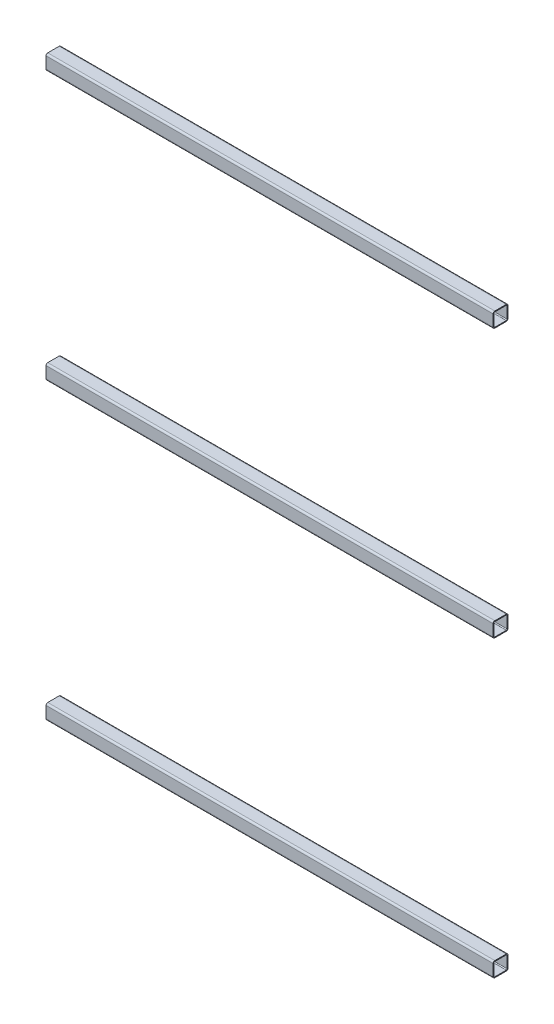
SolidWorks part; units mm, degrees
material "Q235"
ref_plane "Front" through (0, 0, 0) normal (0, 0, 1) x (1, 0, 0)
ref_plane "Top" through (0, 0, 0) normal (0, 1, 0) x (1, 0, 0)
ref_plane "Right" through (0, 0, 0) normal (1, 0, 0) x (0, 0, -1)
sketch "Sketch1" plane through (0, 0, 0) normal (0, 0, 1) x (1, 0, 0)
  line L0 (0, 0) -> (1200, 0)
  line L1 (0, 0) -> (0, 1740)
  line L2 (0, 1740) -> (1200, 1740)
  line L3 (1200, 1740) -> (1200, 0)
  line L4 (0, 1510) -> (1200, 1510)
  line L5 (0, 790) -> (1200, 790)
  line L6 (600, 1740) -> (600, 0)
  dimension "D1" = 1200
  dimension "D2" = 1740
  dimension "D3" = 230
  dimension "D4" = 720
other "Square Tube 40 X 40 X 2.3(1)"
ref_plane "Plane1" through (0, 0, 0) normal (1, 0, 0) x (0, 1, 0)
sketch "Sketch11" plane through (0, 0, 0) normal (1, 0, 0) x (0, 1, 0)
  line L0 (-15.4, -17.7) -> (15.4, -17.7)
  line L1 (-17.7, -15.4) -> (-17.7, 15.4)
  line L2 (15.4, 17.7) -> (-15.4, 17.7)
  line L3 (17.7, 15.4) -> (17.7, -15.4)
  line L4 (-15.4, -20) -> (15.4, -20)
  line L5 (-20, -15.4) -> (-20, 15.4)
  line L6 (15.4, 20) -> (-15.4, 20)
  line L7 (20, 15.4) -> (20, -15.4)
  line L8 (-20, 0) -> (-17.7, 0) construction
  line L9 (-17.7, 0) -> (17.7, 0) construction
  line L10 (17.7, 0) -> (20, 0) construction
  line L12 (0, 20) -> (0, 17.7) construction
  line L13 (0, 17.7) -> (0, -17.7) construction
  line L14 (0, -17.7) -> (0, -20) construction
  arc A0 (20, 15.4) -> (15.4, 20) centre (15.4, 15.4) ccw
  arc A1 (15.4, -20) -> (20, -15.4) centre (15.4, -15.4) ccw
  arc A2 (-20, -15.4) -> (-15.4, -20) centre (-15.4, -15.4) ccw
  arc A3 (-15.4, 20) -> (-20, 15.4) centre (-15.4, 15.4) ccw
  arc A4 (-15.4, 17.7) -> (-17.7, 15.4) centre (-15.4, 15.4) ccw
  arc A5 (17.7, 15.4) -> (15.4, 17.7) centre (15.4, 15.4) ccw
  arc A6 (15.4, -17.7) -> (17.7, -15.4) centre (15.4, -15.4) ccw
  arc A7 (-17.7, -15.4) -> (-15.4, -17.7) centre (-15.4, -15.4) ccw
  point P2 (-20, 20)
  point P33 (-20, -20)
  point P34 (20, -20)
  point P36 (20, 20)
  point P37 (0, 0)
  point P38 (0, 0)
  dimension "D1" = 4.6
  dimension "Thickness" = 2.3
  dimension "V_leg" = 40
  dimension "H_leg" = 40
